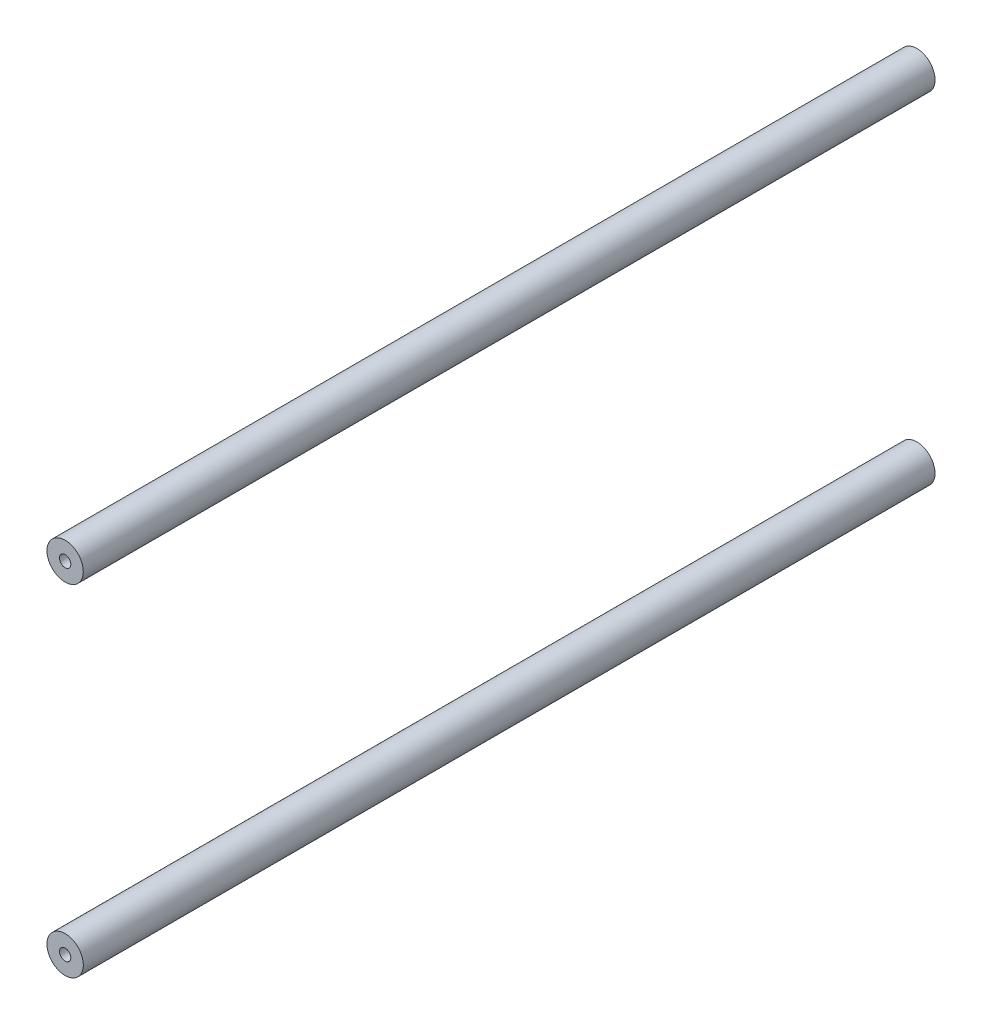
SolidWorks part; units mm, degrees
ref_plane "Front Plane" through (0, 0, 0) normal (0, 0, 1) x (1, 0, 0)
ref_plane "Top Plane" through (0, 0, 0) normal (0, 1, 0) x (1, 0, 0)
ref_plane "Right Plane" through (0, 0, 0) normal (1, 0, 0) x (0, 0, -1)
other "Configuration Table"
sketch "Sketch1" plane through (0, 0, 0) normal (0, 0, 1) x (1, 0, 0)
  line L2 (-88, 90) -> (-57, 90) construction
  line L3 (-90, 57) -> (-90, 88) construction
  line L4 (0, 0) -> (-84.6298, 0) construction
  circle A0 centre (-78, 75) radius 8
  circle A4 centre (-78, -75) radius 8
  dimension "D1" = 16
  dimension "D2" = 15
  dimension "D3" = 12
extrude "Boss-Extrude1" add sketch "Sketch1" along normal blind 375
hole_wizard "M6 Tapped Hole1" positions "Sketch2" profile "Sketch3" tap size "M6" standard "GB" end condition through all
sketch "Sketch2" plane through (0, 0, 0) normal (0, 0, -1) x (-1, 0, 0)
  point P0 (78, 75)
  point P3 (78, -75)
sketch "Sketch3" plane through (-78, 75, 0) normal (1, 0, 0) x (0, 1, 0)
  line L0 (0, 0) -> (0, 375)
  line L1 (0, 375) -> (2.5, 375)
  line L2 (2.5, 375) -> (2.5, 0)
  line L5 (2.5, 0) -> (0, 0)
  line L11 (0, -6.35) -> (0, 107.95) construction
  dimension "通孔螺纹孔钻头直径" = 5
  dimension "通孔螺纹孔钻头深度" = 375
cosmetic thread "Hole thread line1" parameters "D2"=6
cosmetic thread "Hole thread line2" parameters "D2"=6
